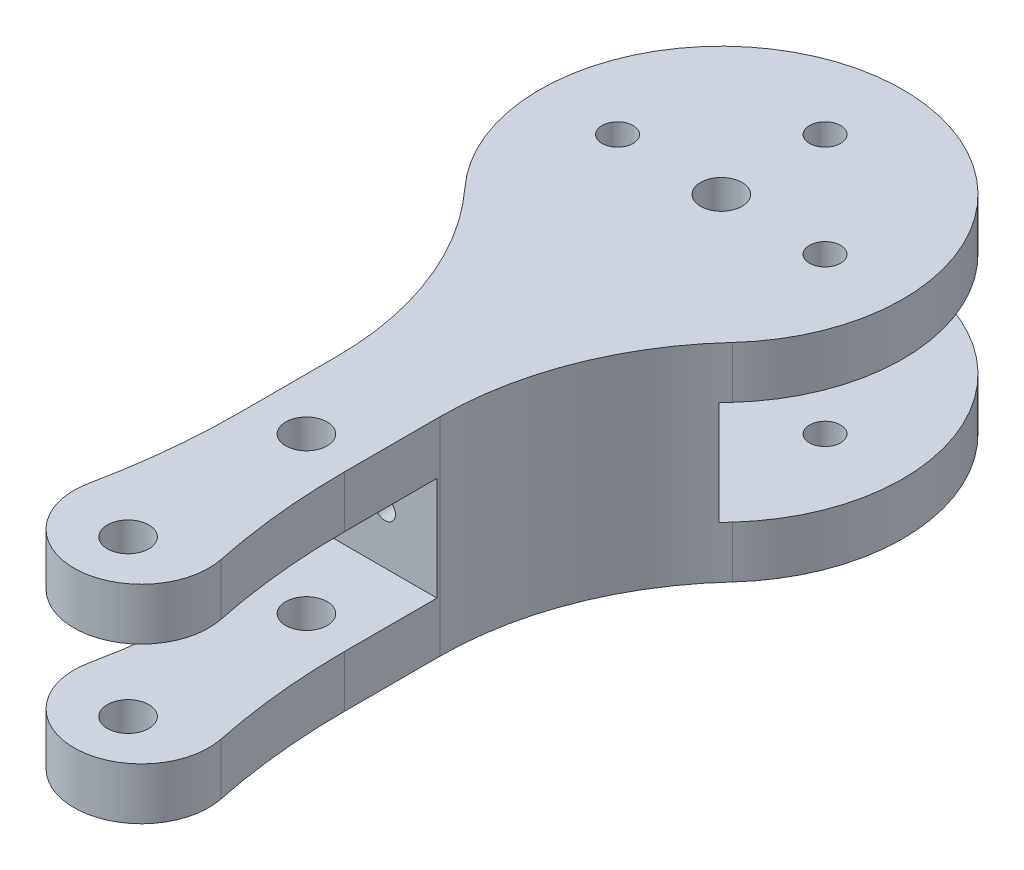
SolidWorks part; units mm, degrees
ref_plane "Front Plane" through (0, 0, 0) normal (0, 0, 1) x (1, 0, 0)
ref_plane "Top Plane" through (0, 0, 0) normal (0, 1, 0) x (1, 0, 0)
ref_plane "Right Plane" through (0, 0, 0) normal (1, 0, 0) x (0, 0, -1)
other "Configuration Table"
sketch "Sketch1" plane through (0, 0, 0) normal (0, 1, 0) x (1, 0, 0)
  line L0 (0, 0) -> (0, -61.3733) construction
  line L1 (-5, -32.1131) -> (-5, -41.3465)
  line L2 (5, -32.1131) -> (5, -41.3465)
  arc A1 (-12.8947, -11.8311) -> (-5, -32.1131) centre (-35, -32.1131) cw
  arc A2 (12.8947, -11.8311) -> (5, -32.1131) centre (35, -32.1131) ccw
  arc A3 (-6.3636, -54.5909) -> (6.3636, -54.5909) centre (0, -55.9153) ccw
  arc A4 (12.8947, -11.8311) -> (-12.8947, -11.8311) centre (0, 0) ccw
  arc A5 (-5, -41.3465) -> (-6.3636, -54.5909) centre (-70, -41.3465) cw
  arc A6 (5, -41.3465) -> (6.3636, -54.5909) centre (70, -41.3465) ccw
  dimension "D1" = 65
  dimension "D3" = 30
  dimension "D4" = 13
  dimension "D2" = 5
extrude "Boss-Extrude1" add sketch "Sketch1" along normal blind 20
sketch "Sketch2" plane through (0, 20, 0) normal (0, 1, 0) x (1, 0, 0)
  circle A0 centre (0, -40) radius 2
  circle A1 centre (0, -57.194) radius 2
  dimension "D2" = 4
  dimension "D3" = 4
  dimension "D1" = 40
extrude "Cut-Extrude1" cut sketch "Sketch2" against normal through all both and the other way through all
sketch "Sketch3" plane through (0, 20, 0) normal (0, 1, 0) x (1, 0, 0)
  circle A0 centre (0, 0) radius 2
  dimension "D1" = 4
extrude "Cut-Extrude2" cut sketch "Sketch3" against normal through all
sketch "Sketch4" plane through (0, 20, 0) normal (0, 1, 0) x (1, 0, 0)
  line L0 (0, 0) -> (-50000, 0) construction
  line L1 (0, 0) -> (0, -50000) construction
  circle A0 centre (-10, 0) radius 1.5
  circle A1 centre (10, 0) radius 1.5
  circle A2 centre (0, 10) radius 1.5
  dimension "D1" = 3
  dimension "D2" = 3
  dimension "D3" = 3
  dimension "D4" = 10
  dimension "D5" = 10
  dimension "D6" = 10
extrude "Cut-Extrude3" cut sketch "Sketch4" against normal through all
sketch "Sketch5" plane through (0, 0, 0) normal (1, 0, 0) x (0, 0, -1)
  line L0 (-62.4153, 15) -> (-32.4153, 15)
  line L1 (-62.4153, 20) -> (-62.4153, 0) construction
  line L2 (-32.4153, 15) -> (-32.4153, 5)
  line L3 (-32.4153, 5) -> (-62.4153, 5)
  line L4 (-62.4153, 5) -> (-62.4153, 15)
  line L5 (-41.3465, 20) -> (-54.5909, 20) construction
  line L6 (-54.5909, 0) -> (-41.3465, 0) construction
  line L7 (-62.4153, 20) -> (17.5, 20) construction
  line L8 (-22.4577, 20) -> (-22.4577, 74.6443) construction
  line L9 (17.5, 5) -> (17.5, 15)
  line L10 (-12.5, 5) -> (17.5, 5)
  line L11 (-12.5, 15) -> (-12.5, 5)
  line L12 (17.5, 15) -> (-12.5, 15)
  dimension "D1" = 5
  dimension "D2" = 5
  dimension "D3" = 30
extrude "Cut-Extrude4" cut sketch "Sketch5" against normal through all both and the other way through all
sketch "Sketch6" plane through (0, 0, 0) normal (0, -1, 0) x (1, 0, 0)
  circle A0 centre (0, 0) radius 6
  dimension "D1" = 12
extrude "Boss-Extrude2" add sketch "Sketch6" along normal blind 5
sketch "Sketch7" plane through (0, 5, 0) normal (0, 1, 0) x (1, 0, 0)
  circle A0 centre (0, 0) radius 2
extrude "Boss-Extrude4" add sketch "Sketch7" along normal up to surface (10 mm away) separate body up to face at (0, 15, -8.5)
sketch "Sketch8" plane through (0, 0, 12.5) normal (0, 0, -1) x (-1, 0, 0)
  circle A0 centre (0, 9.9758) radius 1
  dimension "D1" = 2
extrude "Cut-Extrude5" cut sketch "Sketch8" against normal blind 30
